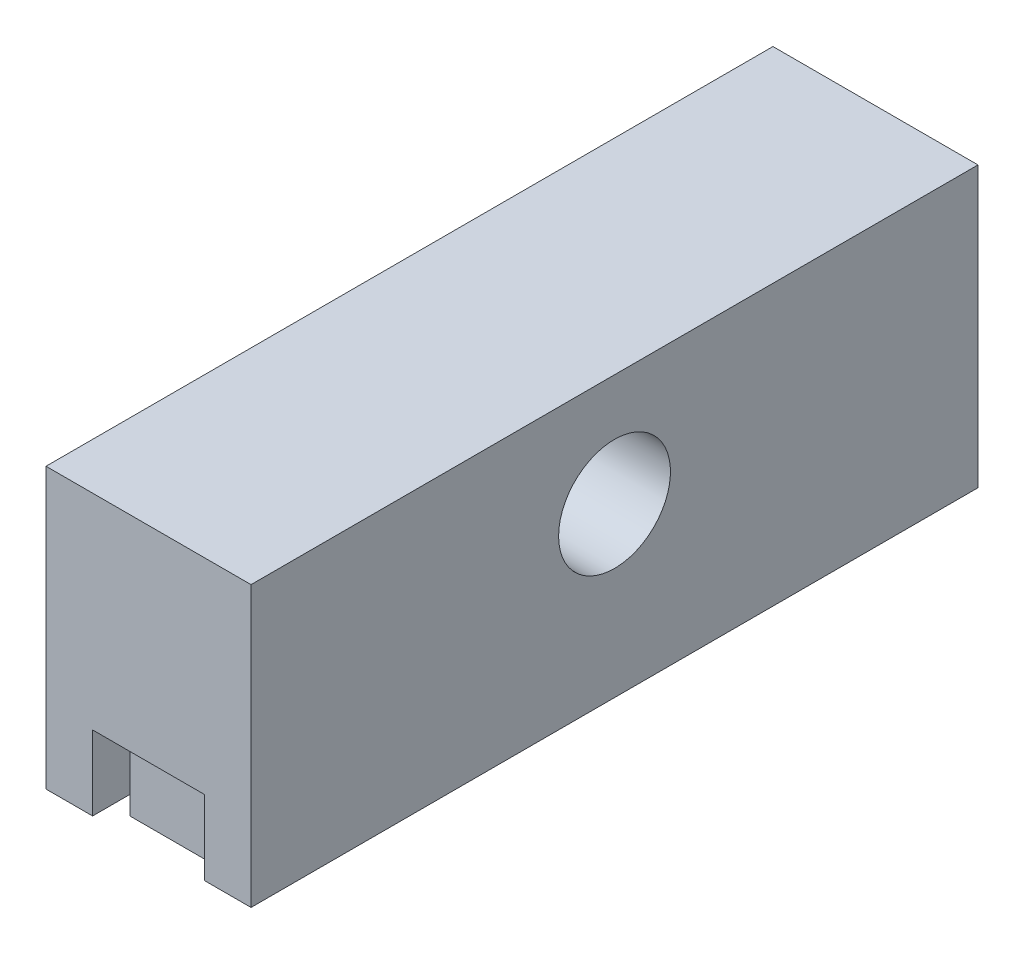
from build123d import *

# Parameters (mm, degrees)
EXTRUDE_1_DEPTH     = 19.5
SKETCH_2_W          = 6
SKETCH_2_H          = 35
EXTRUDE_2_DEPTH     = 5
SKETCH_3_R          = 3
CUT_EXTRUDE_1_DEPTH = 11


with BuildPart() as part:
    # 草图1 → 凸台-拉伸1 (new, symmetric)
    with BuildSketch(Plane.XY):
        Polygon((3, -7.5), (5.5, -7.5), (5.5, 7.5), (-5.5, 7.5), (-5.5, -7.5), (-3, -7.5), (-3, -3.5), (3, -3.5), align=None)
    extrude(amount=EXTRUDE_1_DEPTH, both=True)

    # 草图3 → 切除-拉伸1 (cut)
    with BuildSketch(Plane.ZY.offset(5.5)):
        with Locations((0, 1.5)):
            Circle(SKETCH_3_R)
    extrude(amount=-CUT_EXTRUDE_1_DEPTH, mode=Mode.SUBTRACT)


with BuildPart() as body_2:
    # 草图2 → 凸台-拉伸2 (new body)
    with BuildSketch(Plane.XZ.offset(3.5)):
        Rectangle(SKETCH_2_W, SKETCH_2_H)
    extrude(amount=EXTRUDE_2_DEPTH)


solid = Compound([part.part, body_2.part])
